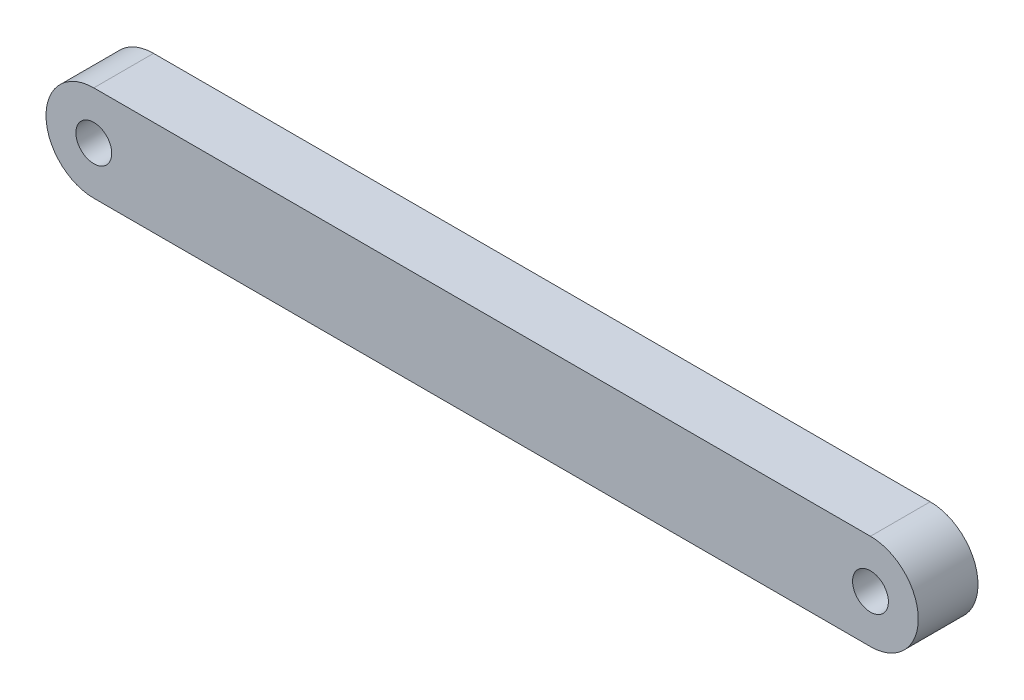
from build123d import *

# Parameters (mm, degrees)
BOSS_EXTRUDE1_DEPTH = 5
SKETCH3_R           = 1.5
CUT_EXTRUDE1_DEPTH  = 38.057387927


with BuildPart() as part:
    # Sketch1 → Boss-Extrude1 (new body)
    with BuildSketch(Plane.XY):
        with BuildLine():
            Line((-32.5, 4), (32.5, 4))
            ThreePointArc((32.5, 4), (36.5, 0), (32.5, -4))
            Line((32.5, -4), (-32.5, -4))
            ThreePointArc((-32.5, -4), (-36.5, 0), (-32.5, 4))
        make_face()
    extrude(amount=BOSS_EXTRUDE1_DEPTH)

    # Sketch3 → Cut-Extrude1 (cut, through all)
    with BuildSketch(Plane.XY.offset(5)):
        with Locations((-32.5, 0)):
            Circle(SKETCH3_R)
        with Locations((32.5, 0)):
            Circle(SKETCH3_R)
    extrude(amount=-CUT_EXTRUDE1_DEPTH, mode=Mode.SUBTRACT)


solid = part.part
